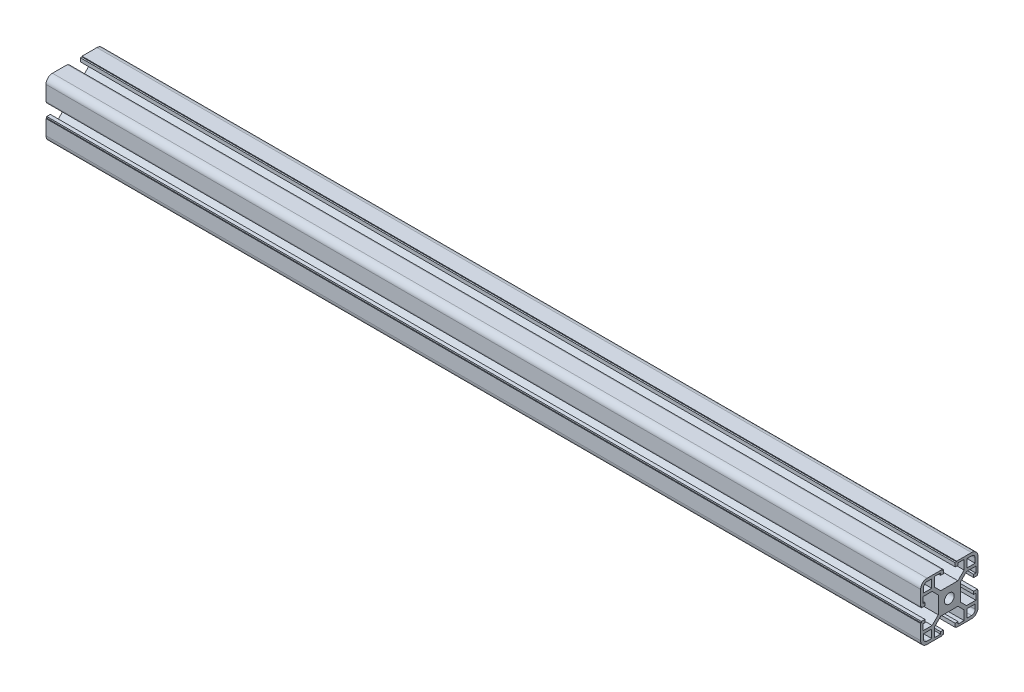
from build123d import *

# Parameters (mm, degrees)
SKETCH1_R                                 = 3.4
ALUMINIUM_PROFILE_40_X_40B_X_R4_5_1_DEPTH = 610


with BuildPart() as part:
    # Sketch1 → Aluminium profile 40 X 40B X R4.5(1) (new body)
    with BuildSketch(Plane.YZ.offset(-984.974958264)):
        with BuildLine():
            Line((-5.1, 20), (-5.1, 19.5))
            Line((-5.1, 19.5), (-4.1, 19.5))
            Line((-4.1, 19.5), (-4.1, 17))
            Line((-4.1, 17), (-6.1, 17))
            Line((-6.1, 17), (-6.1, 18.5))
            Line((-6.1, 18.5), (-10.3, 18.5))
            Line((-10.3, 18.5), (-10.3, 12))
            Line((-10.3, 12), (-6, 7.7))
            Line((-6, 7.7), (6, 7.7))
            Line((6, 7.7), (10.3, 12))
            Line((10.3, 12), (10.3, 18.5))
            Line((10.3, 18.5), (6.1, 18.5))
            Line((6.1, 18.5), (6.1, 17))
            Line((6.1, 17), (4.1, 17))
            Line((4.1, 17), (4.1, 19.5))
            Line((4.1, 19.5), (5.1, 19.5))
            Line((5.1, 19.5), (5.1, 20))
            Line((5.1, 20), (15.5, 20))
            ThreePointArc((15.5, 20), (18.681980515, 18.681980515), (20, 15.5))
            Line((20, 15.5), (20, 5.1))
            Line((20, 5.1), (19.5, 5.1))
            Line((19.5, 5.1), (19.5, 4.1))
            Line((19.5, 4.1), (17, 4.1))
            Line((17, 4.1), (17, 6.1))
            Line((17, 6.1), (18.5, 6.1))
            Line((18.5, 6.1), (18.5, 10.3))
            Line((18.5, 10.3), (12, 10.3))
            Line((12, 10.3), (7.7, 6))
            Line((7.7, 6), (7.7, -6))
            Line((7.7, -6), (12, -10.3))
            Line((12, -10.3), (18.5, -10.3))
            Line((18.5, -10.3), (18.5, -6.1))
            Line((18.5, -6.1), (17, -6.1))
            Line((17, -6.1), (17, -4.1))
            Line((17, -4.1), (19.5, -4.1))
            Line((19.5, -4.1), (19.5, -5.1))
            Line((19.5, -5.1), (20, -5.1))
            Line((20, -5.1), (20, -15.5))
            ThreePointArc((20, -15.5), (18.681980515, -18.681980515), (15.5, -20))
            Line((15.5, -20), (5.1, -20))
            Line((5.1, -20), (5.1, -19.5))
            Line((5.1, -19.5), (4.1, -19.5))
            Line((4.1, -19.5), (4.1, -17))
            Line((4.1, -17), (6.1, -17))
            Line((6.1, -17), (6.1, -18.5))
            Line((6.1, -18.5), (10.3, -18.5))
            Line((10.3, -18.5), (10.3, -12))
            Line((10.3, -12), (6, -7.7))
            Line((6, -7.7), (-6, -7.7))
            Line((-6, -7.7), (-10.3, -12))
            Line((-10.3, -12), (-10.3, -18.5))
            Line((-10.3, -18.5), (-6.1, -18.5))
            Line((-6.1, -18.5), (-6.1, -17))
            Line((-6.1, -17), (-4.1, -17))
            Line((-4.1, -17), (-4.1, -19.5))
            Line((-4.1, -19.5), (-5.1, -19.5))
            Line((-5.1, -19.5), (-5.1, -20))
            Line((-5.1, -20), (-15.5, -20))
            ThreePointArc((-15.5, -20), (-18.681980515, -18.681980515), (-20, -15.5))
            Line((-20, -15.5), (-20, -5.1))
            Line((-20, -5.1), (-19.5, -5.1))
            Line((-19.5, -5.1), (-19.5, -4.1))
            Line((-19.5, -4.1), (-17, -4.1))
            Line((-17, -4.1), (-17, -6.1))
            Line((-17, -6.1), (-18.5, -6.1))
            Line((-18.5, -6.1), (-18.5, -10.3))
            Line((-18.5, -10.3), (-12, -10.3))
            Line((-12, -10.3), (-7.7, -6))
            Line((-7.7, -6), (-7.7, 6))
            Line((-7.7, 6), (-12, 10.3))
            Line((-12, 10.3), (-18.5, 10.3))
            Line((-18.5, 10.3), (-18.5, 6.1))
            Line((-18.5, 6.1), (-17, 6.1))
            Line((-17, 6.1), (-17, 4.1))
            Line((-17, 4.1), (-19.5, 4.1))
            Line((-19.5, 4.1), (-19.5, 5.1))
            Line((-19.5, 5.1), (-20, 5.1))
            Line((-20, 5.1), (-20, 15.5))
            ThreePointArc((-20, 15.5), (-18.681980515, 18.681980515), (-15.5, 20))
            Line((-15.5, 20), (-5.1, 20))
        make_face()
        Circle(SKETCH1_R, mode=Mode.SUBTRACT)
        with BuildLine():
            Line((12.3, 18), (15.5, 18))
            ThreePointArc((15.5, 18), (17.267766953, 17.267766953), (18, 15.5))
            Line((18, 15.5), (18, 12.3))
            Line((18, 12.3), (12.3, 12.3))
            Line((12.3, 12.3), (12.3, 18))
        make_face(mode=Mode.SUBTRACT)
        with BuildLine():
            Line((-15.5, 18), (-12.3, 18))
            Line((-12.3, 18), (-12.3, 12.3))
            Line((-12.3, 12.3), (-18, 12.3))
            Line((-18, 12.3), (-18, 15.5))
            ThreePointArc((-18, 15.5), (-17.267766953, 17.267766953), (-15.5, 18))
        make_face(mode=Mode.SUBTRACT)
        with BuildLine():
            Line((-18, -12.3), (-12.3, -12.3))
            Line((-12.3, -12.3), (-12.3, -18))
            Line((-12.3, -18), (-15.5, -18))
            ThreePointArc((-15.5, -18), (-17.267766953, -17.267766953), (-18, -15.5))
            Line((-18, -15.5), (-18, -12.3))
        make_face(mode=Mode.SUBTRACT)
        with BuildLine():
            Line((12.3, -12.3), (18, -12.3))
            Line((18, -12.3), (18, -15.5))
            ThreePointArc((18, -15.5), (17.267766953, -17.267766953), (15.5, -18))
            Line((15.5, -18), (12.3, -18))
            Line((12.3, -18), (12.3, -12.3))
        make_face(mode=Mode.SUBTRACT)
    extrude(amount=ALUMINIUM_PROFILE_40_X_40B_X_R4_5_1_DEPTH)


solid = part.part
